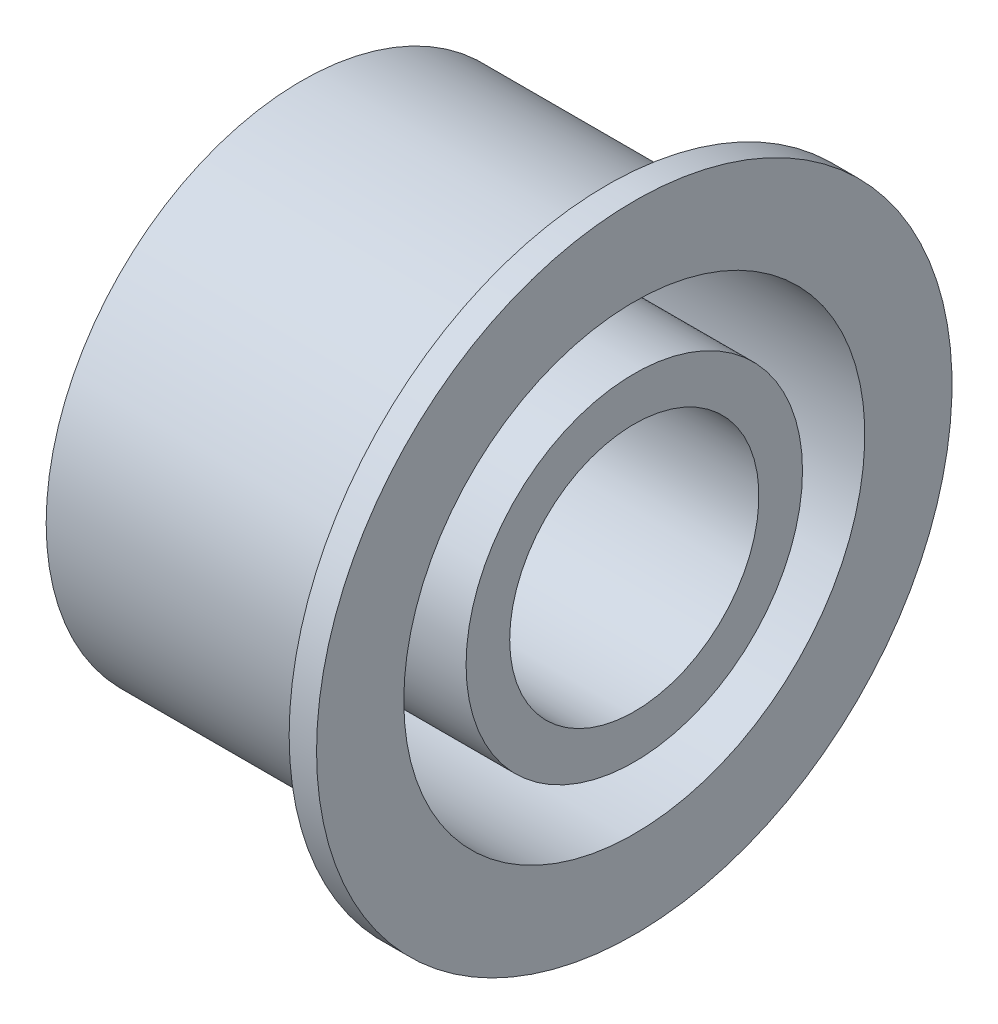
SolidWorks part; units mm, degrees
ref_plane "前视基准面" through (0, 0, 0) normal (0, 0, 1) x (1, 0, 0)
ref_plane "上视基准面" through (0, 0, 0) normal (0, 1, 0) x (1, 0, 0)
ref_plane "右视基准面" through (0, 0, 0) normal (1, 0, 0) x (0, 0, -1)
sketch "草图1" plane through (0, 0, 0) normal (0, 0, 1) x (1, 0, 0)
  line L0 (0, 0) -> (86.1435, 0) construction
  line L1 (25.3, 25.5) -> (25.3, 20.5)
  line L2 (25.3, 20.5) -> (0.8, 20.5)
  line L3 (0.8, 20.5) -> (0.8, 13.5)
  line L4 (0.8, 13.5) -> (0, 13.5)
  line L5 (0, 13.5) -> (0, 10)
  line L6 (0, 10) -> (27.5, 10)
  line L7 (27.5, 10) -> (27.5, 13.5)
  line L8 (27.5, 13.5) -> (4.3, 13.5)
  line L9 (4.3, 13.5) -> (4.3, 18.5)
  line L10 (4.3, 18.5) -> (27.5, 18.5)
  line L11 (27.5, 18.5) -> (27.5, 25.5)
  line L12 (27.5, 25.5) -> (25.3, 25.5)
  line L13 (0, 0) -> (0, 32.4564) construction
  dimension "D1" = 25.5
  dimension "D2" = 20.5
  dimension "D3" = 2.2
  dimension "D4" = 24.5
  dimension "D5" = 27.5
  dimension "D6" = 10
  dimension "D7" = 2
  dimension "D8" = 13.5
  dimension "D9" = 3.5
revolve "旋转1" add sketch "草图1" angle 360 about L0
